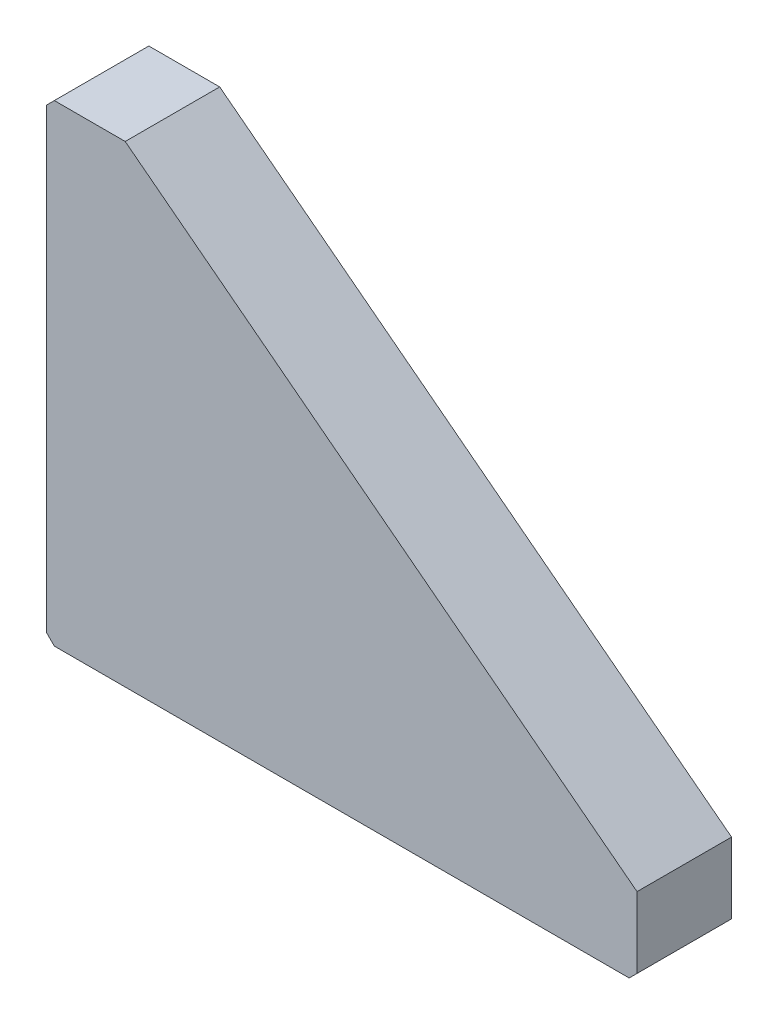
from build123d import *

# Parameters (mm, degrees)
SKETCH1_W             = 75
SKETCH1_H             = 60
BOSS_EXTRUDE1_DEPTH   = 6
CUT_EXTRUDE1_DEPTH    = 50.5
M6_TAPPED_HOLE1_D     = 5
M6_TAPPED_HOLE1_DEPTH = 12
M6_TAPPED_HOLE1_TIP   = 1.502151548
M6_TAPPED_HOLE2_D     = 5
M6_TAPPED_HOLE2_DEPTH = 15
M6_TAPPED_HOLE2_TIP   = 1.502151548
CHAMFER1_SIZE         = 1


with BuildPart() as part:
    # Sketch1 → Boss-Extrude1 (new, symmetric)
    with BuildSketch(Plane.XY):
        Rectangle(SKETCH1_W, SKETCH1_H)
    extrude(amount=BOSS_EXTRUDE1_DEPTH, both=True)

    # Sketch2 → Cut-Extrude1 (cut, through all)
    with BuildSketch(Plane.XY.offset(6)):
        Polygon((-27.5, 30), (37.5, -20), (37.5, 30), align=None)
    extrude(amount=-CUT_EXTRUDE1_DEPTH, mode=Mode.SUBTRACT)

    # M6 Tapped Hole1
    with Locations(Plane.ZY.offset(37.5)):
        with Locations((0, 20), (0, -15)):
            Hole(M6_TAPPED_HOLE1_D / 2, depth=M6_TAPPED_HOLE1_DEPTH)
            with Locations((0, 0, -(M6_TAPPED_HOLE1_DEPTH + M6_TAPPED_HOLE1_TIP / 2))):  # 118° drill point
                Cone(0, M6_TAPPED_HOLE1_D / 2, M6_TAPPED_HOLE1_TIP, mode=Mode.SUBTRACT)

    # M6 Tapped Hole2
    with Locations(Plane(origin=(0, -30, 0), x_dir=(-1, 0, 0), z_dir=(0, -1, 0))):
        with Locations((22.5, 0), (-27.5, 0)):
            Hole(M6_TAPPED_HOLE2_D / 2, depth=M6_TAPPED_HOLE2_DEPTH)
            with Locations((0, 0, -(M6_TAPPED_HOLE2_DEPTH + M6_TAPPED_HOLE2_TIP / 2))):  # 118° drill point
                Cone(0, M6_TAPPED_HOLE2_D / 2, M6_TAPPED_HOLE2_TIP, mode=Mode.SUBTRACT)

    # Chamfer1
    chamfer1_edges = [part.edges().sort_by_distance(p)[0] for p in [
        (37.5, -30, 0),
        (-37.5, -30, 0),
        (-37.5, 30, 0),
    ]]
    chamfer(chamfer1_edges, length=CHAMFER1_SIZE)


solid = part.part
